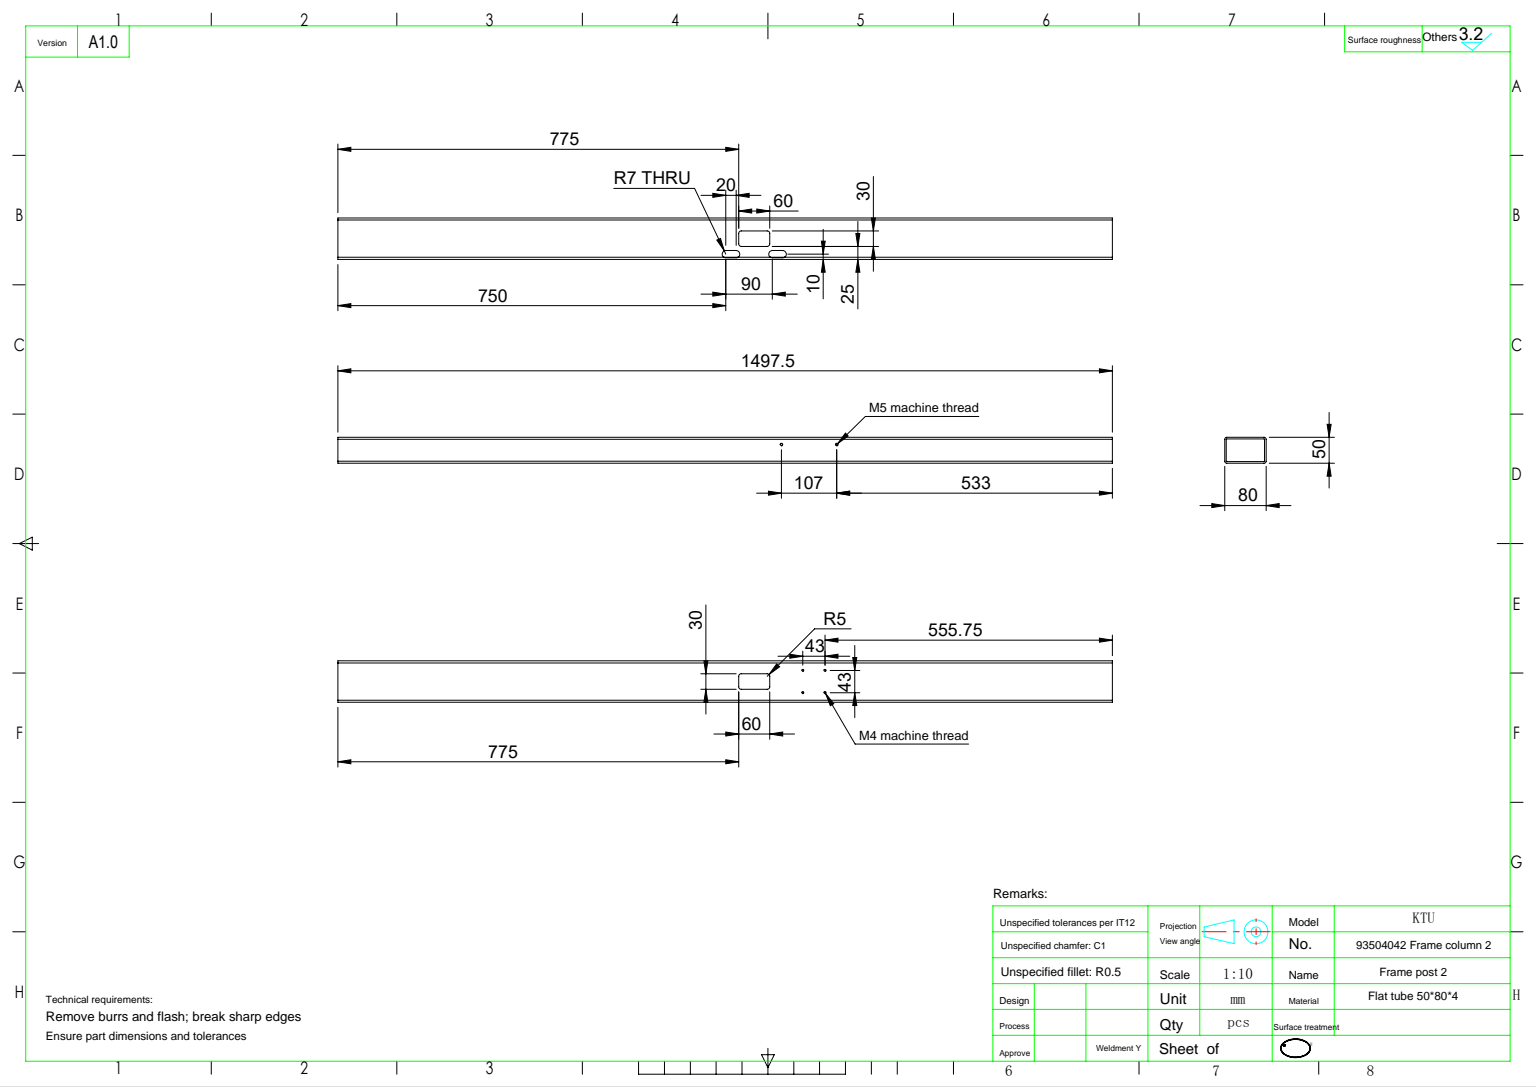
from build123d import *

# Parameters (mm, degrees)
EXTRUDE_1_DEPTH     = 748.75
CUT_EXTRUDE_2_DEPTH = 10
CUT_EXTRUDE_3_DEPTH = 752.482909092
SKETCH_6_R          = 1.65
CUT_EXTRUDE_4_DEPTH = 10
SKETCH_7_R          = 2.1
CUT_EXTRUDE_5_DEPTH = 10


with BuildPart() as part:
    # 草图1 → 拉伸-薄壁1 (new, symmetric)
    with BuildSketch(Plane.XY):
        with BuildLine():
            Line((-36, 25), (36, 25))
            ThreePointArc((36, 25), (38.828427125, 23.828427125), (40, 21))
            Line((40, 21), (40, -21))
            ThreePointArc((40, -21), (38.828427125, -23.828427125), (36, -25))
            Line((36, -25), (-36, -25))
            ThreePointArc((-36, -25), (-38.828427125, -23.828427125), (-40, -21))
            Line((-40, -21), (-40, 21))
            ThreePointArc((-40, 21), (-38.828427125, 23.828427125), (-36, 25))
        make_face()
        with BuildLine():
            Line((-36, 22), (36, 22))
            ThreePointArc((36, 22), (36.707106781, 21.707106781), (37, 21))
            Line((37, 21), (37, -21))
            ThreePointArc((37, -21), (36.707106781, -21.707106781), (36, -22))
            Line((36, -22), (-36, -22))
            ThreePointArc((-36, -22), (-36.707106781, -21.707106781), (-37, -21))
            Line((-37, -21), (-37, 21))
            ThreePointArc((-37, 21), (-36.707106781, 21.707106781), (-36, 22))
        make_face(mode=Mode.SUBTRACT)
    extrude(amount=EXTRUDE_1_DEPTH, both=True)

    # 草图4 → 切除-拉伸2 (cut)
    with BuildSketch(Plane.XZ.offset(25)):
        with BuildLine():
            Line((23, 91.25), (23, 111.25))
            ThreePointArc((23, 111.25), (30, 118.25), (37, 111.25))
            Line((37, 111.25), (37, 91.25))
            ThreePointArc((37, 91.25), (30, 84.25), (23, 91.25))
        make_face()
        with BuildLine():
            Line((23, 1.25), (23, 21.25))
            ThreePointArc((23, 21.25), (30, 28.25), (37, 21.25))
            Line((37, 21.25), (37, 1.25))
            ThreePointArc((37, 1.25), (30, -5.75), (23, 1.25))
        make_face()
    extrude(amount=-CUT_EXTRUDE_2_DEPTH, mode=Mode.SUBTRACT)

    # 草图5 → 切除-拉伸3 (cut, through all)
    with BuildSketch(Plane.XZ.offset(25)):
        with BuildLine():
            Line((-10, 26.25), (10, 26.25))
            ThreePointArc((10, 26.25), (13.535533906, 27.714466094), (15, 31.25))
            Line((15, 31.25), (15, 81.25))
            ThreePointArc((15, 81.25), (13.535533906, 84.785533906), (10, 86.25))
            Line((10, 86.25), (-10, 86.25))
            ThreePointArc((-10, 86.25), (-13.535533906, 84.785533906), (-15, 81.25))
            Line((-15, 81.25), (-15, 31.25))
            ThreePointArc((-15, 31.25), (-13.535533906, 27.714466094), (-10, 26.25))
        make_face()
    extrude(amount=-CUT_EXTRUDE_3_DEPTH, mode=Mode.SUBTRACT)

    # 草图6 → 切除-拉伸4 (cut)
    with BuildSketch(Plane(origin=(0, 25, 0), x_dir=(1, 0, 0), z_dir=(0, 1, 0))):
        with Locations(Location((-21.5, -150, 0), (0, 0, 270))):
            Circle(SKETCH_6_R)
        with Locations(Location((-21.5, -193, 0), (0, 0, 270))):
            Circle(SKETCH_6_R)
        with Locations(Location((21.5, -150, 0), (0, 0, 270))):
            Circle(SKETCH_6_R)
        with Locations(Location((21.5, -193, 0), (0, 0, 270))):
            Circle(SKETCH_6_R)
    extrude(amount=-CUT_EXTRUDE_4_DEPTH, mode=Mode.SUBTRACT)

    # 草图7 → 切除-拉伸5 (cut)
    with BuildSketch(Plane.ZY.offset(40)):
        with Locations(Location((108.75, 11, 0), (0, 0, 270))):
            Circle(SKETCH_7_R)
        with Locations(Location((215.75, 11, 0), (0, 0, 270))):
            Circle(SKETCH_7_R)
    extrude(amount=-CUT_EXTRUDE_5_DEPTH, mode=Mode.SUBTRACT)


solid = part.part
